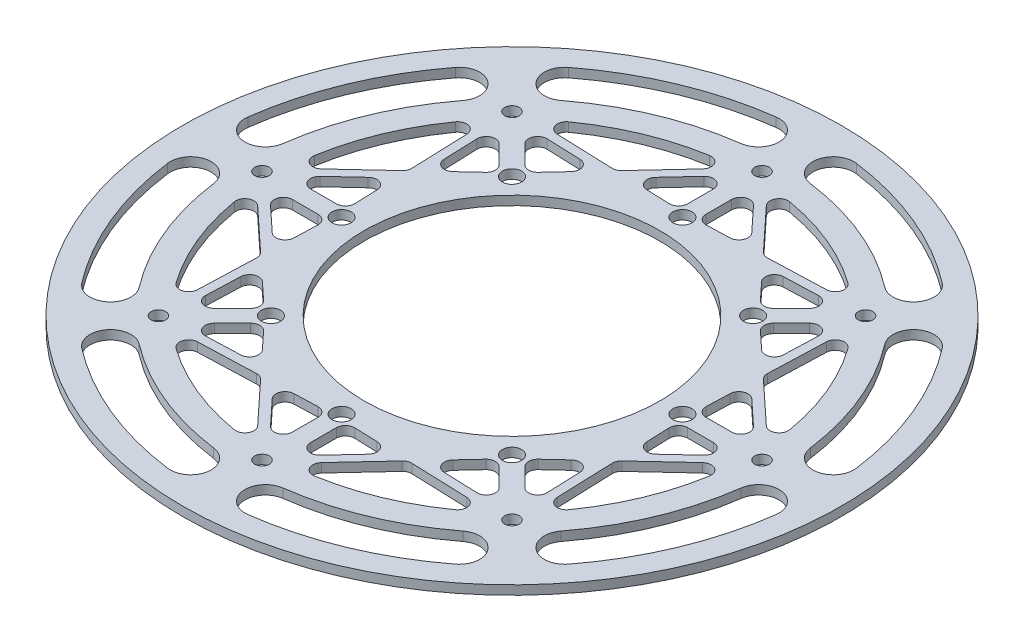
from build123d import *

# Parameters (mm, degrees)
SKETCH_1_R                       = 72.5
SKETCH_1_R_2                     = 32.5
SKETCH_1_R_3                     = 1.5999999999999988
SKETCH_1_R_4                     = 1.6000000000000127
SKETCH_1_R_5                     = 1.599999999999998
SKETCH_1_R_6                     = 1.5999999999999974
SKETCH_1_R_7                     = 1.5999999999999963
SKETCH_1_R_8                     = 2.0999999999999996
SKETCH_1_R_9                     = 2.100000000000001
SKETCH_1_R_10                    = 2.0999999999999974
EXTRUDE_1_DEPTH                  = 2
CUT_EXTRUDE_1_DEPTH              = 103.54998781082327
FILLET_1_R                       = 2
PATTERN_CIRCULAR_1_COUNT         = 8
FILLET_1_OF_PATTERN_CIRCULAR_1_R = 2


with BuildPart() as part:
    # 草图1 → 凸台-拉伸1 (new body)
    with BuildSketch(Plane(origin=(0, 0, 0), x_dir=(1, 0, 0), z_dir=(0, 1, 0))):
        with Locations(Location((0, 0, 0), (0, 0, 270))):
            Circle(SKETCH_1_R)
        with Locations(Location((0, 0, 0), (0, 0, 270))):
            Circle(SKETCH_1_R_2, mode=Mode.SUBTRACT)
        with Locations(Location((0, 55, 0), (0, 0, 270))):
            Circle(SKETCH_1_R_3, mode=Mode.SUBTRACT)
        with Locations(Location((38.890872965260115, 38.890872965260115, 0), (0, 0, 270))):
            Circle(SKETCH_1_R_4, mode=Mode.SUBTRACT)
        with Locations(Location((55, 3.47e-15, 0), (0, 0, 270))):
            Circle(SKETCH_1_R_5, mode=Mode.SUBTRACT)
        with Locations(Location((38.890872965260115, -38.89087296526011, 0), (0, 0, 270))):
            Circle(SKETCH_1_R_6, mode=Mode.SUBTRACT)
        with Locations(Location((6.94e-15, -55, 0), (0, 0, 270))):
            Circle(SKETCH_1_R_7, mode=Mode.SUBTRACT)
        with Locations(Location((-38.89087296526011, -38.89087296526012, 0), (0, 0, 270))):
            Circle(SKETCH_1_R_6, mode=Mode.SUBTRACT)
        with Locations(Location((-55, -1.008e-14, 0), (0, 0, 270))):
            Circle(SKETCH_1_R_5, mode=Mode.SUBTRACT)
        with Locations(Location((-38.89087296526012, 38.89087296526011, 0), (0, 0, 270))):
            Circle(SKETCH_1_R_6, mode=Mode.SUBTRACT)
        with Locations(Location((0, 37.50000000000001, 0), (0, 0, 270))):
            Circle(SKETCH_1_R_8, mode=Mode.SUBTRACT)
        with Locations(Location((26.516504294495537, 26.51650429449554, 0), (0, 0, 270))):
            Circle(SKETCH_1_R_9, mode=Mode.SUBTRACT)
        with Locations(Location((37.50000000000001, 2.6e-15, 0), (0, 0, 270))):
            Circle(SKETCH_1_R_10, mode=Mode.SUBTRACT)
        with Locations(Location((26.51650429449554, -26.516504294495537, 0), (0, 0, 270))):
            Circle(SKETCH_1_R_9, mode=Mode.SUBTRACT)
        with Locations(Location((4.77e-15, -37.50000000000001, 0), (0, 0, 270))):
            Circle(SKETCH_1_R_8, mode=Mode.SUBTRACT)
        with Locations(Location((-26.516504294495537, -26.516504294495544, 0), (0, 0, 270))):
            Circle(SKETCH_1_R_9, mode=Mode.SUBTRACT)
        with Locations(Location((-37.50000000000001, -6.94e-15, 0), (0, 0, 270))):
            Circle(SKETCH_1_R_10, mode=Mode.SUBTRACT)
        with Locations(Location((-26.516504294495544, 26.51650429449553, 0), (0, 0, 270))):
            Circle(SKETCH_1_R_9, mode=Mode.SUBTRACT)
        with BuildLine():
            ThreePointArc((-8.810517974853264, 66.92252814273222), (-25.831131684643175, 62.361868444512), (-41.09139645808817, 53.551350469658736))
            ThreePointArc((-41.09139645808817, 53.551350469658736), (-41.922060058859536, 47.24183400780896), (-35.612543597009754, 46.41117040703758))
            ThreePointArc((-35.612543597009754, 46.41117040703758), (-22.38698079335743, 54.04695265191042), (-7.635782244872831, 57.999524390367945))
            ThreePointArc((-7.635782244872831, 57.999524390367945), (-3.76164823368089, 63.04839413154031), (-8.810517974853264, 66.92252814273222))
        make_face(mode=Mode.SUBTRACT)
        with BuildLine():
            ThreePointArc((41.091396458088816, 53.551350469658225), (25.831131684643946, 62.361868444511686), (8.81051797485408, 66.92252814273212))
            ThreePointArc((8.81051797485408, 66.92252814273212), (3.761648233681676, 63.048394131540256), (7.635782244873538, 57.99952439036785))
            ThreePointArc((7.635782244873538, 57.99952439036785), (22.3869807933581, 54.04695265191016), (35.61254359701033, 46.41117040703715))
            ThreePointArc((35.61254359701033, 46.41117040703715), (41.922060058860126, 47.24183400780845), (41.091396458088816, 53.551350469658225))
        make_face(mode=Mode.SUBTRACT)
        with BuildLine():
            ThreePointArc((66.92252814273223, 8.810517974853253), (62.36186844451201, 25.831131684643175), (53.551350469658736, 41.09139645808817))
            ThreePointArc((53.551350469658736, 41.09139645808817), (47.24183400780896, 41.922060058859536), (46.411170407037595, 35.612543597009754))
            ThreePointArc((46.411170407037595, 35.612543597009754), (54.04695265191044, 22.386980793357427), (57.99952439036797, 7.635782244872823))
            ThreePointArc((57.99952439036797, 7.635782244872823), (63.048394131540306, 3.761648233680912), (66.92252814273223, 8.810517974853253))
        make_face(mode=Mode.SUBTRACT)
        with BuildLine():
            ThreePointArc((53.55135046965822, -41.091396458088816), (62.361868444511686, -25.831131684643932), (66.92252814273212, -8.81051797485407))
            ThreePointArc((66.92252814273212, -8.81051797485407), (63.048394131540256, -3.761648233681669), (57.99952439036785, -7.635782244873532))
            ThreePointArc((57.99952439036785, -7.635782244873532), (54.04695265191015, -22.38698079335809), (46.41117040703714, -35.61254359701033))
            ThreePointArc((46.41117040703714, -35.61254359701033), (47.241834007808436, -41.922060058860126), (53.55135046965822, -41.091396458088816))
        make_face(mode=Mode.SUBTRACT)
        with BuildLine():
            ThreePointArc((8.810517974853255, -66.92252814273222), (25.831131684643168, -62.361868444512), (41.09139645808818, -53.55135046965873))
            ThreePointArc((41.09139645808818, -53.55135046965873), (41.92206005885954, -47.241834007808954), (35.61254359700976, -46.41117040703758))
            ThreePointArc((35.61254359700976, -46.41117040703758), (22.386980793357424, -54.04695265191042), (7.635782244872825, -57.99952439036795))
            ThreePointArc((7.635782244872825, -57.99952439036795), (3.7616482336808996, -63.048394131540306), (8.810517974853255, -66.92252814273222))
        make_face(mode=Mode.SUBTRACT)
        with BuildLine():
            ThreePointArc((-41.091396458088816, -53.55135046965823), (-25.83113168464392, -62.36186844451169), (-8.810517974854065, -66.92252814273215))
            ThreePointArc((-8.810517974854065, -66.92252814273215), (-3.7616482336816404, -63.04839413154026), (-7.635782244873527, -57.99952439036787))
            ThreePointArc((-7.635782244873527, -57.99952439036787), (-22.38698079335808, -54.04695265191017), (-35.61254359701033, -46.41117040703716))
            ThreePointArc((-35.61254359701033, -46.41117040703716), (-41.9220600588601, -47.24183400780845), (-41.091396458088816, -53.55135046965823))
        make_face(mode=Mode.SUBTRACT)
        with BuildLine():
            ThreePointArc((-66.92252814273222, -8.81051797485326), (-62.36186844451199, -25.831131684643204), (-53.55135046965873, -41.09139645808818))
            ThreePointArc((-53.55135046965873, -41.09139645808818), (-47.241834007808954, -41.92206005885954), (-46.41117040703758, -35.61254359700976))
            ThreePointArc((-46.41117040703758, -35.61254359700976), (-54.04695265191042, -22.386980793357456), (-57.99952439036795, -7.635782244872829))
            ThreePointArc((-57.99952439036795, -7.635782244872829), (-63.048394131540306, -3.761648233680905), (-66.92252814273222, -8.81051797485326))
        make_face(mode=Mode.SUBTRACT)
        with BuildLine():
            ThreePointArc((-53.551350469658225, 41.091396458088816), (-62.36186844451169, 25.83113168464392), (-66.92252814273212, 8.810517974854083))
            ThreePointArc((-66.92252814273212, 8.810517974854083), (-63.048394131540256, 3.7616482336816794), (-57.99952439036785, 7.635782244873542))
            ThreePointArc((-57.99952439036785, 7.635782244873542), (-54.04695265191016, 22.386980793358077), (-46.41117040703715, 35.61254359701033))
            ThreePointArc((-46.41117040703715, 35.61254359701033), (-47.24183400780845, 41.922060058860126), (-53.551350469658225, 41.091396458088816))
        make_face(mode=Mode.SUBTRACT)
    extrude(amount=EXTRUDE_1_DEPTH)

    # 草图2 → 切除-拉伸1 (cut, symmetric)
    with BuildSketch(Plane(origin=(0, 2, 0), x_dir=(1, 0, 0), z_dir=(0, 1, 0))):
        Polygon((13.542813764109777, 38.9849774608073), (1.9999999999999987, 51.38403589731881), (2.000000000000002, 38.57216626930041), align=None)
        with BuildLine():
            ThreePointArc((35.051441007977395, 39.75420082537543), (20.28222191534894, 48.965615223098524), (3.325353357172003, 52.895576611375965))
            Line((3.3253533571729292, 52.895576611377635), (16.187280783175485, 39.07955280468365))
            Line((16.18728078317549, 39.079552804683644), (35.051441007977566, 39.754200825376046))
        make_face()
        Polygon((34.919786665354025, 37.74821379010021), (17.990326477993023, 37.14275737589009), (25.860426771704237, 28.68885389645043), align=None)
    cut_extrude_1 = extrude(amount=CUT_EXTRUDE_1_DEPTH, both=True, mode=Mode.SUBTRACT)

    # 圆角1
    fillet_1_edges = [part.edges().sort_by_distance(p)[0] for p in [
        (25.860426771704237, 1, -28.688853896450425),
        (17.990326477993023, 1, -37.1427573758901),
        (34.919786665354025, 1, -37.74821379010021),
        (35.05144100797748, 1, -39.75420082537574),
        (16.18728078317549, 1, -39.079552804683644),
        (3.3253533571724656, 1, -52.895576611376804),
        (1.9999999999999996, 1, -51.38403589731881),
        (13.542813764109777, 1, -38.9849774608073),
        (2.000000000000002, 1, -38.57216626930041),
    ]]
    fillet(fillet_1_edges, radius=FILLET_1_R)

    # 阵列(圆周)1: 切除-拉伸1 ×8 about axis
    pattern_circular_1_axis = Axis((-2.572e-14, 0, -1.032e-14), (0, 1, 0))
    for i in range(1, PATTERN_CIRCULAR_1_COUNT):
        add(cut_extrude_1.rotate(pattern_circular_1_axis, i * 360 / PATTERN_CIRCULAR_1_COUNT), mode=Mode.SUBTRACT)

    # 圆角1 of 阵列(圆周)1
    fillet_1_of_pattern_circular_1_edges = [part.edges().sort_by_distance(p)[0] for p in [
        (-1.9999999999999967, 1, -38.572166269300425),
        (-13.542813764109775, 1, -38.984977460807336),
        (-1.9999999999999931, 1, -51.38403589731883),
        (-3.325353357173914, 1, -52.895576611376164),
        (-16.18728078317549, 1, -39.079552804683665),
        (-35.05144100797897, 1, -39.7542008253752),
        (-34.91978666535402, 1, -37.74821379010023),
        (-17.990326477993015, 1, -37.14275737589011),
        (-25.860426771704237, 1, -28.688853896450453),
        (-28.68885389645044, 1, -25.860426771704272),
        (-37.14275737589011, 1, -17.99032647799306),
        (-37.74821379010022, 1, -34.91978666535406),
        (-39.754200825375754, 1, -35.051441007977516),
        (-39.07955280468366, 1, -16.187280783175527),
        (-52.89557661137682, 1, -3.3253533571725047),
        (-51.384035897318824, 1, -2.0000000000000386),
        (-38.984977460807315, 1, -13.542813764109814),
        (-38.572166269300425, 1, -2.0000000000000404),
        (-38.57216626930044, 1, 1.9999999999999607),
        (-38.98497746080735, 1, 13.54281376410974),
        (-51.384035897318846, 1, 1.9999999999999571),
        (-52.89557661137618, 1, 3.3253533571738774),
        (-39.07955280468368, 1, 16.187280783175453),
        (-39.754200825375214, 1, 35.05144100797894),
        (-37.748213790100245, 1, 34.91978666535398),
        (-37.14275737589013, 1, 17.99032647799298),
        (-28.688853896450468, 1, 25.8604267717042),
        (-25.86042677170429, 1, 28.6888538964504),
        (-17.990326477993076, 1, 37.14275737589008),
        (-34.91978666535408, 1, 37.74821379010018),
        (-35.05144100797754, 1, 39.75420082537571),
        (-16.18728078317554, 1, 39.07955280468362),
        (-3.325353357172524, 1, 52.89557661137678),
        (-2.0000000000000573, 1, 51.38403589731879),
        (-13.542813764109834, 1, 38.98497746080728),
        (-2.0000000000000586, 1, 38.57216626930039),
        (1.9999999999999416, 1, 38.57216626930041),
        (13.542813764109722, 1, 38.984977460807315),
        (1.999999999999938, 1, 51.38403589731881),
        (3.3253533571738587, 1, 52.89557661137614),
        (16.18728078317544, 1, 39.079552804683644),
        (35.05144100797892, 1, 39.754200825375186),
        (34.91978666535397, 1, 37.748213790100216),
        (17.990326477992966, 1, 37.1427573758901),
        (25.860426771704187, 1, 28.688853896450436),
        (28.688853896450386, 1, 25.860426771704255),
        (37.14275737589006, 1, 17.990326477993044),
        (37.748213790100166, 1, 34.919786665354046),
        (39.7542008253757, 1, 35.0514410079775),
        (39.07955280468361, 1, 16.18728078317551),
        (52.89557661137677, 1, 3.325353357172491),
        (51.384035897318775, 1, 2.0000000000000244),
        (38.984977460807265, 1, 13.5428137641098),
        (38.572166269300375, 1, 2.000000000000025),
        (38.57216626930039, 1, -1.9999999999999742),
        (38.9849774608073, 1, -13.542813764109754),
        (51.384035897318796, 1, -1.9999999999999707),
        (52.89557661137613, 1, -3.325353357173891),
        (39.07955280468363, 1, -16.187280783175467),
        (39.75420082537517, 1, -35.05144100797896),
        (37.7482137901002, 1, -34.919786665354),
        (37.14275737589008, 1, -17.990326477992994),
        (28.68885389645042, 1, -25.86042677170422),
    ]]
    fillet(fillet_1_of_pattern_circular_1_edges, radius=FILLET_1_OF_PATTERN_CIRCULAR_1_R)


solid = part.part
